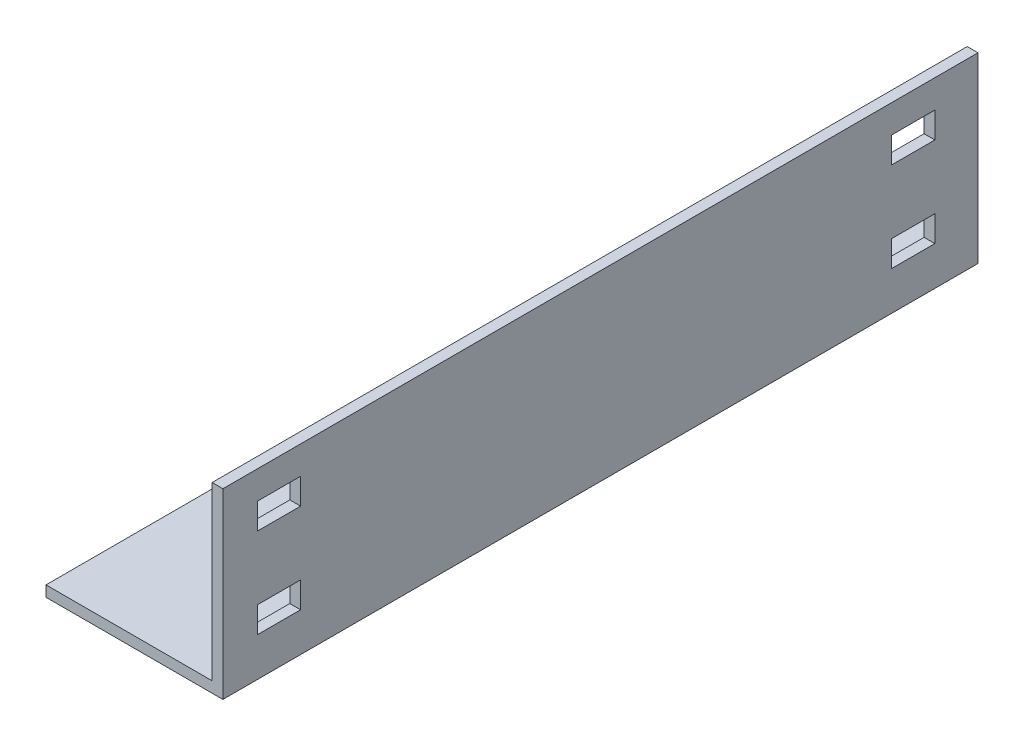
SolidWorks part; units mm, degrees
ref_plane "前视基准面" through (0, 0, 0) normal (0, 0, 1) x (1, 0, 0)
ref_plane "上视基准面" through (0, 0, 0) normal (0, 1, 0) x (1, 0, 0)
ref_plane "右视基准面" through (0, 0, 0) normal (1, 0, 0) x (0, 0, -1)
sketch "草图1" plane through (0, 0, 0) normal (0, 0, 1) x (1, 0, 0)
  line L0 (-295.1404, 27.0191) -> (-295.1404, 2.0191)
  line L1 (114.8596, 2.0191) -> (114.8596, 425)
  line L2 (114.8596, 425) -> (89.8596, 425)
  line L3 (89.8596, 425) -> (89.8596, 27.0191)
  line L4 (89.8596, 27.0191) -> (-295.1404, 27.0191)
  line L5 (-295.1404, 2.0191) -> (114.8596, 2.0191)
extrude "凸台-拉伸1" add sketch "草图1" along normal mid plane 1750
sketch "草图2" plane through (0, 0, 0) normal (1, 0, 0) x (0, 0, -1)
  line L0 (775, 300) -> (675, 300)
  line L2 (675, 300) -> (675, 360)
  line L3 (775, 360) -> (675, 360)
  line L5 (775, 360) -> (775, 300)
  line L8 (-795, 300) -> (-795, 360)
  line L10 (-795, 300) -> (-695, 300)
  line L11 (-795, 360) -> (-695, 360)
  line L12 (-695, 360) -> (-695, 300)
  line L15 (775, 92.0191) -> (675, 92.0191)
  line L16 (675, 92.0191) -> (675, 152.0191)
  line L17 (675, 152.0191) -> (775, 152.0191)
  line L18 (775, 152.0191) -> (775, 92.0191)
  line L23 (-795, 92.0191) -> (-795, 152.0191)
  line L24 (-795, 152.0191) -> (-695, 152.0191)
  line L25 (-695, 152.0191) -> (-695, 92.0191)
  line L26 (-695, 92.0191) -> (-795, 92.0191)
extrude "切除-拉伸2" cut sketch "草图2" along normal through all
